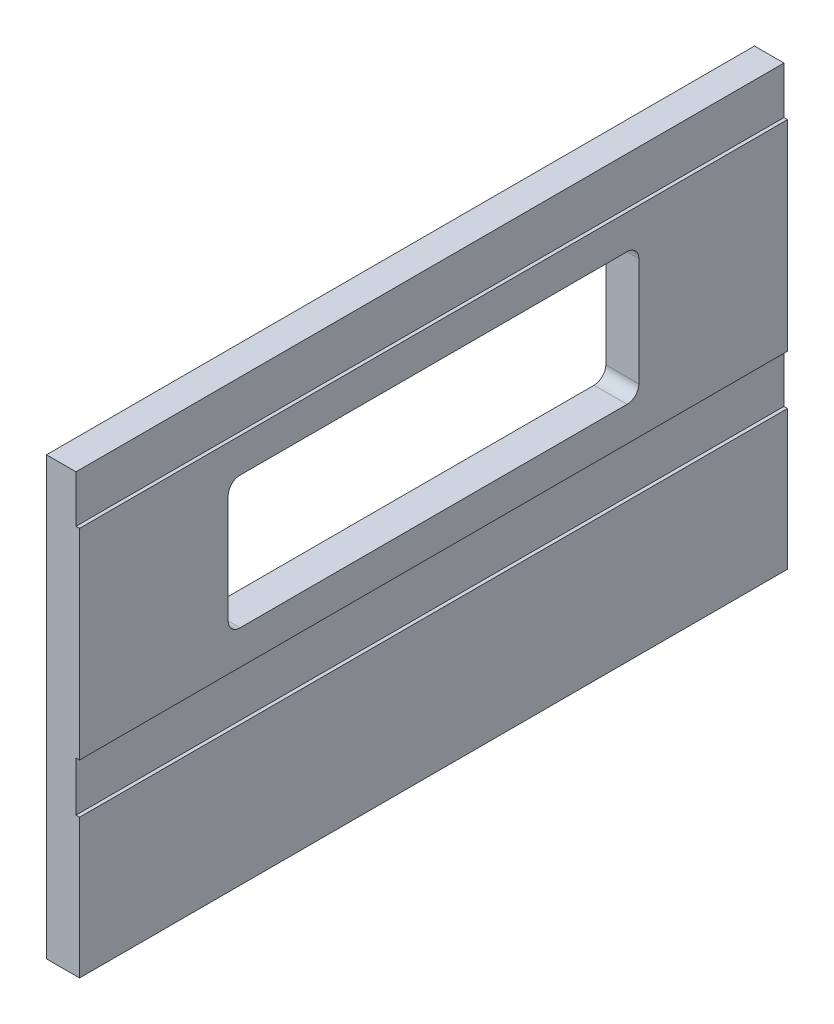
from build123d import *

# Parameters (mm, degrees)
SKETCH_1_W          = 14
SKETCH_1_H          = 185
EXTRUDE_1_DEPTH     = 150
SKETCH_2_W          = 300
SKETCH_2_H          = 20
SKETCH_2_H_2        = 21
CUT_EXTRUDE_1_DEPTH = 1.5
CUT_EXTRUDE_2_REACH = 240.581
SKETCH_3_W          = 174
SKETCH_3_H          = 56
FILLET_1_R          = 5


with BuildPart() as part:
    # 草图1 → 凸台-拉伸1 (new, symmetric)
    with BuildSketch(Plane.XY):
        with Locations((7, 92.5)):
            Rectangle(SKETCH_1_W, SKETCH_1_H)
    extrude(amount=EXTRUDE_1_DEPTH, both=True)

    # 草图2 → 切除-拉伸1 (cut)
    with BuildSketch(Plane(origin=(14, 0, 0), x_dir=(0, 0, -1), z_dir=(1, 0, 0))):
        with Locations((0, 175)):
            Rectangle(SKETCH_2_W, SKETCH_2_H)
        with Locations((0, 69.5)):
            Rectangle(SKETCH_2_W, SKETCH_2_H_2)
    extrude(amount=-CUT_EXTRUDE_1_DEPTH, mode=Mode.SUBTRACT)

    # 草图3 → 切除-拉伸2 (cut, up to next)
    with BuildSketch(Plane(origin=(14, 0, 0), x_dir=(0, 0, -1), z_dir=(1, 0, 0)), mode=Mode.PRIVATE) as cut_extrude_2_sk1:
        with Locations((0, 122.5)):
            Rectangle(SKETCH_3_W, SKETCH_3_H)
    cut_extrude_2_tool1 = extrude(cut_extrude_2_sk1.sketch, amount=-CUT_EXTRUDE_2_REACH, mode=Mode.PRIVATE) & part.part
    add(cut_extrude_2_tool1.solids().sort_by_distance((14, 122.5, 0))[0], mode=Mode.SUBTRACT)

    # 圆角1
    fillet_1_edges = [part.edges().sort_by_distance(p)[0] for p in [
        (7, 150.5, -87),
        (7, 94.5, -87),
        (7, 94.5, 87),
        (7, 150.5, 87),
    ]]
    fillet(fillet_1_edges, radius=FILLET_1_R)


solid = part.part
